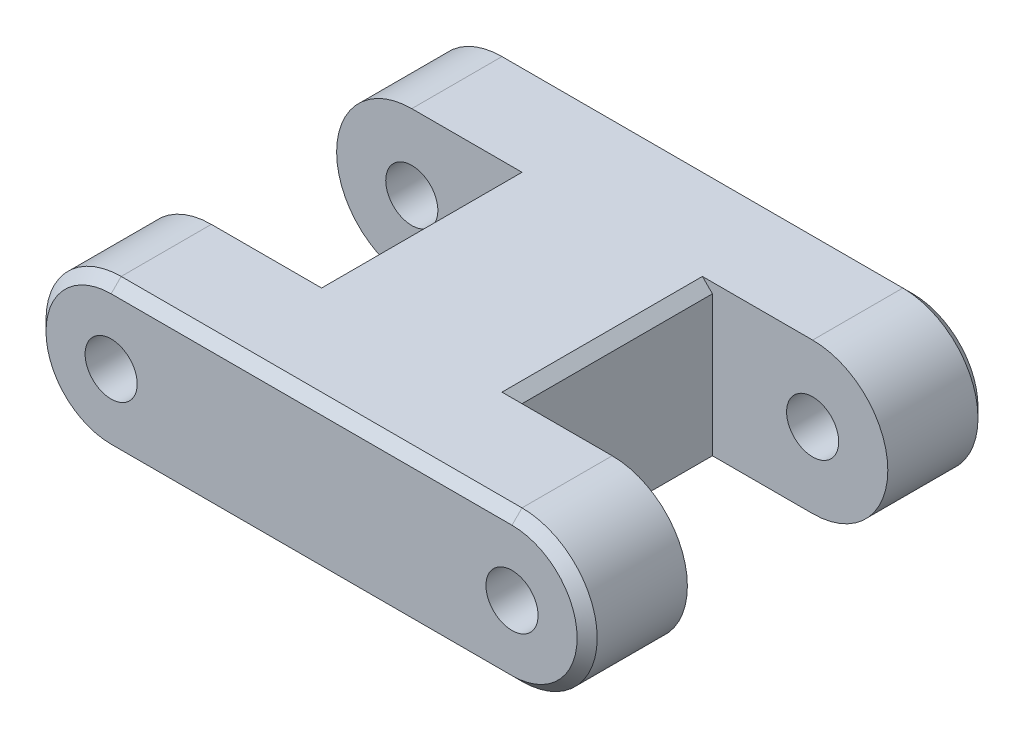
from build123d import *

# Parameters (mm, degrees)
SKETCH1_R           = 2.6
BOSS_EXTRUDE1_DEPTH = 5
SKETCH2_W           = 20
SKETCH2_H           = 15
BOSS_EXTRUDE2_DEPTH = 20
SKETCH3_R           = 2.6
BOSS_EXTRUDE3_DEPTH = 10
CHAMFER1_SIZE       = 1


with BuildPart() as part:
    # Sketch1 → Boss-Extrude1 (new, symmetric)
    with BuildSketch(Plane.XY):
        with BuildLine():
            Line((0, -7.5), (-40, -7.5))
            ThreePointArc((-40, -7.5), (-47.5, 0), (-40, 7.5))
            Line((-40, 7.5), (0, 7.5))
            ThreePointArc((0, 7.5), (7.5, 0), (0, -7.5))
        make_face()
        Circle(SKETCH1_R, mode=Mode.SUBTRACT)
        with Locations((-40, 0)):
            Circle(SKETCH1_R, mode=Mode.SUBTRACT)
    extrude(amount=BOSS_EXTRUDE1_DEPTH, both=True)

    # Sketch2 → Boss-Extrude2 (add)
    with BuildSketch(Plane(origin=(0, 0, -5), x_dir=(-1, 0, 0), z_dir=(0, 0, -1))):
        with Locations((20, 0)):
            Rectangle(SKETCH2_W, SKETCH2_H)
    extrude(amount=BOSS_EXTRUDE2_DEPTH)

    # Sketch3 → Boss-Extrude3 (add)
    with BuildSketch(Plane(origin=(0, 0, -25), x_dir=(-1, 0, 0), z_dir=(0, 0, -1))):
        with BuildLine():
            Line((0, 7.5), (40, 7.5))
            ThreePointArc((40, 7.5), (47.5, 0), (40, -7.5))
            Line((40, -7.5), (0, -7.5))
            ThreePointArc((0, -7.5), (-7.5, 0), (0, 7.5))
        make_face()
        with Locations(Location((0, 0, 0), (0, 0, 180))):
            Circle(SKETCH3_R, mode=Mode.SUBTRACT)
        with Locations(Location((40, 0, 0), (0, 0, 180))):
            Circle(SKETCH3_R, mode=Mode.SUBTRACT)
    extrude(amount=BOSS_EXTRUDE3_DEPTH)

    # Chamfer1
    chamfer1_edges = [part.edges().sort_by_distance(p)[0] for p in [
        (-47.5, 0, 5),
        (-20, -7.5, 5),
        (-30, 7.5, -15),
        (-10, 7.5, -15),
        (7.5, 0, -35),
        (-20, -7.5, -35),
        (-47.5, 0, -35),
        (-20, 7.5, -35),
        (7.5, 0, 5),
        (-20, 7.5, 5),
    ]]
    chamfer(chamfer1_edges, length=CHAMFER1_SIZE)


solid = part.part
